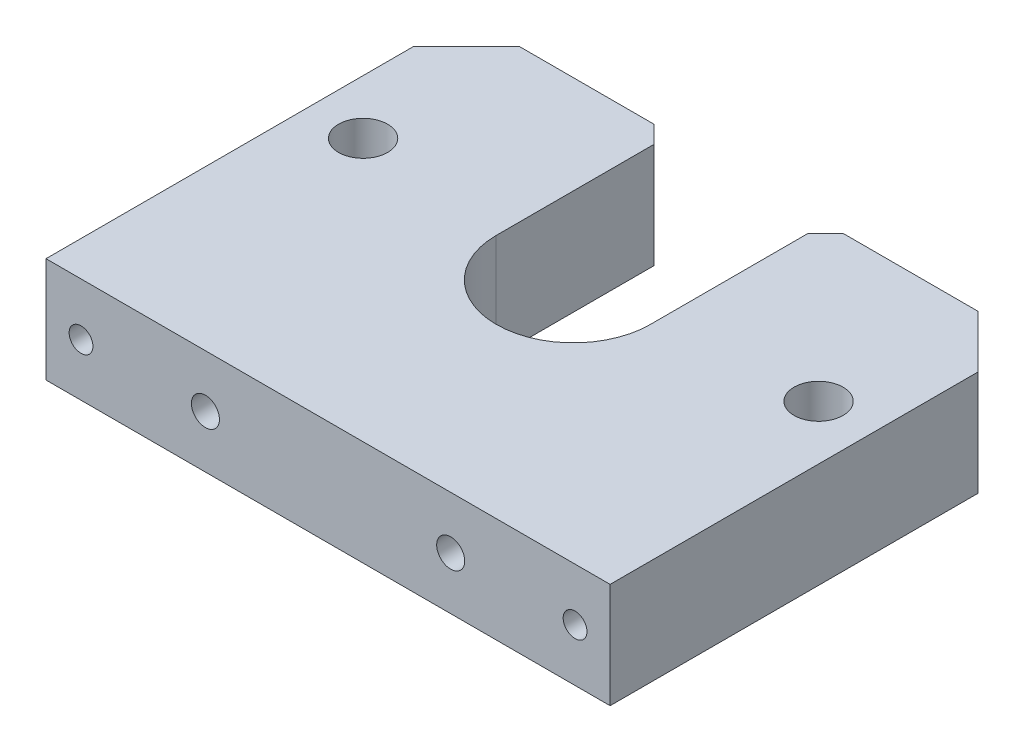
from build123d import *

# Parameters (mm, degrees)
SKETCH1_W             = 161
SKETCH1_H             = 120
BOSS_EXTRUDE1_DEPTH   = 30
CUT_EXTRUDE1_DEPTH    = 105.786688086
M16_TAPPED_HOLE1_D    = 14
M8_TAPPED_HOLE1_D     = 6.8
M8_TAPPED_HOLE1_DEPTH = 19.75
M8_TAPPED_HOLE1_TIP   = 2.042926105
SKETCH7_R             = 4
CUT_EXTRUDE2_DEPTH    = 15
CHAMFER1_SIZE         = 15
CHAMFER2_SIZE         = 5


with BuildPart() as part:
    # Sketch1 → Boss-Extrude1 (new body)
    with BuildSketch(Plane(origin=(0, 0, 0), x_dir=(1, 0, 0), z_dir=(0, 1, 0))):
        Rectangle(SKETCH1_W, SKETCH1_H)
    extrude(amount=BOSS_EXTRUDE1_DEPTH)

    # Sketch2 → Cut-Extrude1 (cut, through all)
    with BuildSketch(Plane(origin=(0, 30, 0), x_dir=(1, 0, 0), z_dir=(0, 1, 0))):
        with BuildLine():
            Line((-22, 10), (-22, 60))
            Line((-22, 60), (22, 60))
            Line((22, 60), (22, 10))
            ThreePointArc((22, 10), (0, -12), (-22, 10))
        make_face()
    extrude(amount=-CUT_EXTRUDE1_DEPTH, mode=Mode.SUBTRACT)

    # M16 Tapped Hole1 (through all)
    with Locations(Plane(origin=(0, 30, 0), x_dir=(-1, 0, 0), z_dir=(0, 1, 0))):
        with Locations((65, -15), (-65, -15)):
            Hole(M16_TAPPED_HOLE1_D / 2)

    # M8 Tapped Hole1
    with Locations(Plane.XY.offset(60)):
        with Locations((70.5, 15), (-70.5, 15)):
            Hole(M8_TAPPED_HOLE1_D / 2, depth=M8_TAPPED_HOLE1_DEPTH)
            with Locations((0, 0, -(M8_TAPPED_HOLE1_DEPTH + M8_TAPPED_HOLE1_TIP / 2))):  # 118° drill point
                Cone(0, M8_TAPPED_HOLE1_D / 2, M8_TAPPED_HOLE1_TIP, mode=Mode.SUBTRACT)

    # Sketch7 → Cut-Extrude2 (cut)
    with BuildSketch(Plane.XY.offset(60)):
        with Locations((-35, 15)):
            Circle(SKETCH7_R)
        with Locations((35, 15)):
            Circle(SKETCH7_R)
    extrude(amount=-CUT_EXTRUDE2_DEPTH, mode=Mode.SUBTRACT)

    # Chamfer1
    chamfer1_edges = [part.edges().sort_by_distance(p)[0] for p in [
        (-80.5, 15, -60),
        (80.5, 15, -60),
    ]]
    chamfer(chamfer1_edges, length=CHAMFER1_SIZE)

    # Chamfer2
    chamfer2_edges = [part.edges().sort_by_distance(p)[0] for p in [
        (-22, 15, -60),
        (22, 15, -60),
    ]]
    chamfer(chamfer2_edges, length=CHAMFER2_SIZE)


solid = part.part
